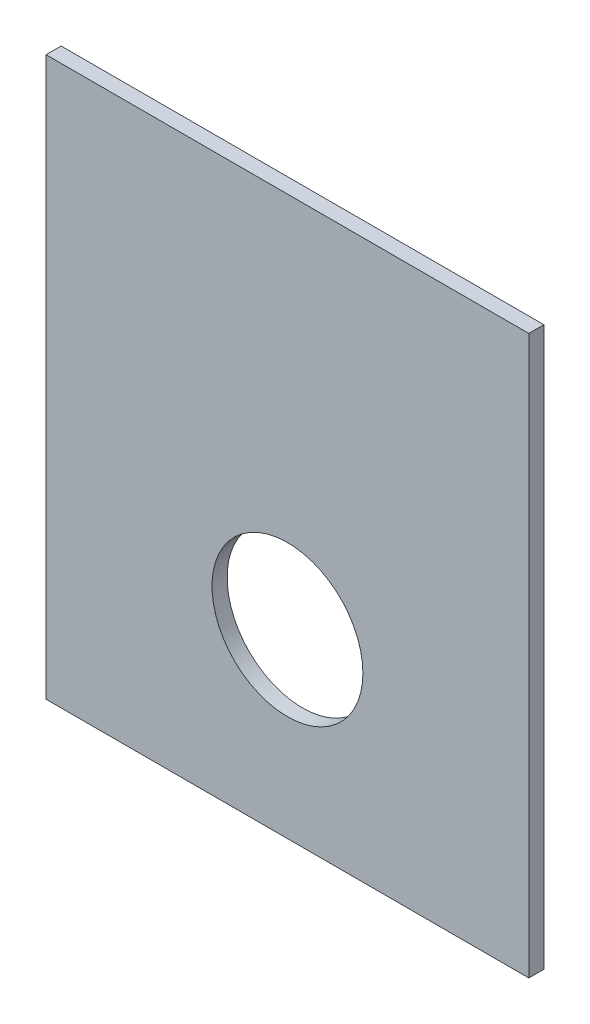
SolidWorks part; units mm, degrees
ref_plane "Front Plane" through (0, 0, 0) normal (0, 0, 1) x (1, 0, 0)
ref_plane "Top Plane" through (0, 0, 0) normal (0, 1, 0) x (1, 0, 0)
ref_plane "Right Plane" through (0, 0, 0) normal (1, 0, 0) x (0, 0, -1)
sketch "Sketch1" plane through (0, 0, 0) normal (0, 0, 1) x (1, 0, 0)
  line L1 (0, 0) -> (320, 0)
  line L2 (0, 0) -> (0, 370)
  line L3 (0, 370) -> (320, 370)
  line L4 (320, 0) -> (320, 370)
  circle A0 centre (160, 120) radius 50
  dimension "D5" = 100
  dimension "D1" = 370
  dimension "D2" = 320
  dimension "D3" = 160
  dimension "D4" = 120
extrude "Boss-Extrude1" add sketch "Sketch1" along normal blind 10
